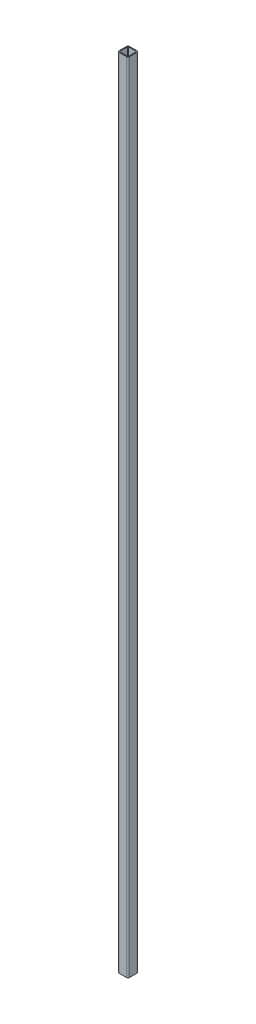
SolidWorks part; units mm, degrees
material "Q235B"
ref_plane "Front Plane" through (0, 0, 0) normal (0, 0, 1) x (1, 0, 0)
ref_plane "Top Plane" through (0, 0, 0) normal (0, 1, 0) x (1, 0, 0)
ref_plane "Right Plane" through (0, 0, 0) normal (1, 0, 0) x (0, 0, -1)
sketch "Sketch1" plane through (0, 0, 0) normal (0, 0, 1) x (1, 0, 0)
  line L0 (0, 0) -> (0, 9220)
  dimension "D1" = 9220
other "Cold-formed hollow square steel (GB/T 6728-2002) 120×120×10(1)"
ref_plane "Plane1" through (0, 0, 0) normal (0, 1, 0) x (-1, 0, 0)
sketch "Sketch12" plane through (0, 0, 0) normal (0, 1, 0) x (-1, 0, 0)
  line L0 (-44, -50) -> (44, -50)
  line L1 (-50, -44) -> (-50, 44)
  line L2 (44, 50) -> (-44, 50)
  line L3 (50, 44) -> (50, -44)
  line L4 (-44, -60) -> (44, -60)
  line L5 (-60, -44) -> (-60, 44)
  line L6 (44, 60) -> (-44, 60)
  line L7 (60, 44) -> (60, -44)
  arc A0 (60, 44) -> (44, 60) centre (44, 44) ccw
  arc A1 (44, -60) -> (60, -44) centre (44, -44) ccw
  arc A2 (-60, -44) -> (-44, -60) centre (-44, -44) ccw
  arc A3 (-44, 60) -> (-60, 44) centre (-44, 44) ccw
  arc A4 (-44, 50) -> (-50, 44) centre (-44, 44) ccw
  arc A5 (50, 44) -> (44, 50) centre (44, 44) ccw
  arc A6 (44, -50) -> (50, -44) centre (44, -44) ccw
  arc A7 (-50, -44) -> (-44, -50) centre (-44, -44) ccw
  point P0 (-60, 0)
  point P1 (60, 0)
  point P2 (0, 60)
  point P3 (0, -60)
  point P4 (0, 0)
  point P5 (-60, -60)
  point P6 (60, -60)
  point P7 (60, 60)
  point P8 (-60, 60)
  point P33 (0, 0)
  dimension "D1" = 16
  dimension "D2" = 120
  dimension "D3" = 10
